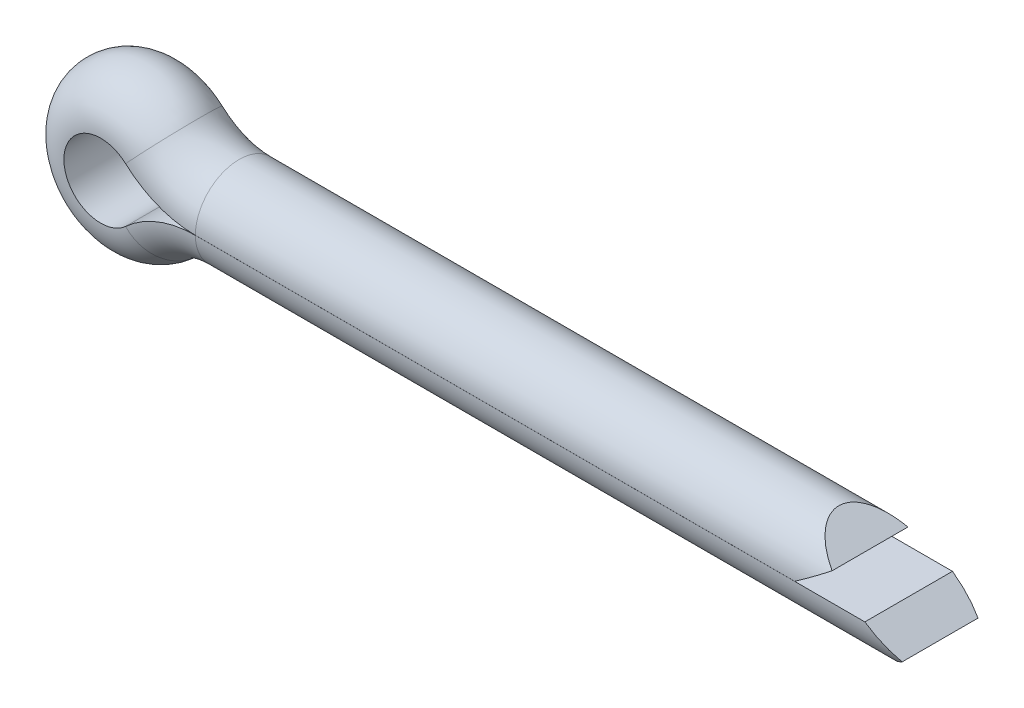
SolidWorks part; units mm, degrees
material "Q235A"
ref_plane "Front" through (0, 0, 0) normal (0, 0, 1) x (1, 0, 0)
ref_plane "Top" through (0, 0, 0) normal (0, 1, 0) x (1, 0, 0)
ref_plane "Right" through (0, 0, 0) normal (1, 0, 0) x (0, 0, -1)
sketch "Sketch2" plane through (0, 0, 0) normal (0, 0, 1) x (1, 0, 0)
  line L0 (36, 2.5) -> (0, 2.5)
  line L1 (0, -2.5) -> (40, -2.5)
  line L2 (0, 0) -> (49.7718, 0) construction
  line L3 (0, 0) -> (0, 16.5256) construction
  line L4 (-10, 0) -> (-10, 14.2137) construction
  arc A0 (0, 2.5) -> (-2.2922, 3.3914) centre (0, 5.8929) cw
  arc A1 (-2.2922, 3.3914) -> (-2.2922, -3.3914) centre (-5.4, 0) ccw
  arc A2 (-2.2922, -3.3914) -> (0, -2.5) centre (0, -5.8929) cw
  dimension "c" = 9.2
  dimension "Diameter" = 5
  dimension "b" = 10
  dimension "l" = 36
  dimension "a" = 4
ref_plane "SectionPlane" through (36, 0, 0) normal (1, 0, 0) x (0, 0, -1)
sketch "Sketch1" plane through (36, 0, 0) normal (1, 0, 0) x (0, 0, -1)
  line L1 (-2.5, 0.002) -> (2.5, 0.002)
  arc A0 (2.5, 0.002) -> (-2.5, 0.002) centre (0, 0) ccw
  dimension "D1" = 0.002
  dimension "Diameter" = 5
sweep "Body" add profiles "Sketch1" path "Sketch2"
sketch "Sketch3" plane through (0, 0, 0) normal (0, 0, 1) x (1, 0, 0)
  line L0 (0, 0) -> (0, 16.2682) construction
  line L1 (0, 0) -> (75.9079, 0) construction
  line L2 (0, 0) -> (40, 0) construction
  line L3 (36, 1.251) -> (34.2105, 2.51)
  line L4 (36, 0.002) -> (36, 2.5) construction
  line L6 (36, 1.251) -> (34.2049, 0)
  line L7 (40, -1.251) -> (38.2049, 0)
  line L8 (40, -2.5) -> (40, -0.002) construction
  line L9 (40, -1.251) -> (38.2105, -2.51)
  line L10 (38.2049, 0) -> (34.2049, 0)
  line L11 (34.2105, 2.51) -> (40.01, 2.51)
  line L12 (40.01, 2.51) -> (40.01, -2.51)
  line L13 (40.01, -2.51) -> (38.2105, -2.51)
  line L14 (36, 2.5) -> (0, 2.5) construction
  dimension "D1" = 0.01
  dimension "D2" = 0.01
  dimension "D3" = 70
  dimension "D4" = 70
extrude "ConeCut" cut sketch "Sketch3" against normal through all and the other way through all
